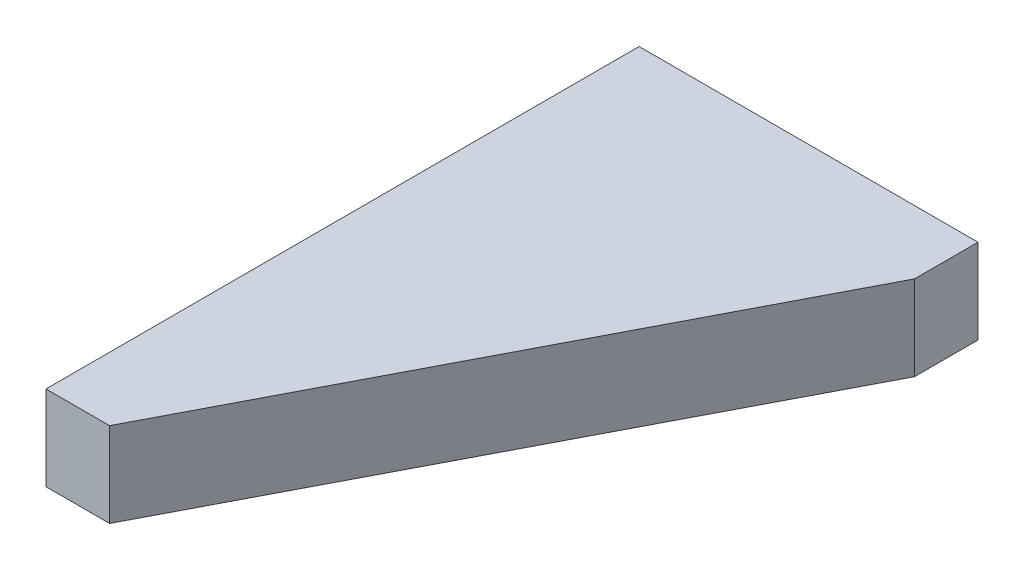
SolidWorks part; units mm, degrees
ref_plane "前视基准面" through (0, 0, 0) normal (0, 0, 1) x (1, 0, 0)
ref_plane "上视基准面" through (0, 0, 0) normal (0, 1, 0) x (1, 0, 0)
ref_plane "右视基准面" through (0, 0, 0) normal (1, 0, 0) x (0, 0, -1)
sketch "草图1" plane through (0, 0, 0) normal (0, 1, 0) x (1, 0, 0)
  line L1 (0, 0) -> (200, 0)
  line L2 (0, 0) -> (0, 140)
  line L3 (0, 140) -> (200, 140)
  line L4 (200, 0) -> (200, 140)
  dimension "D1" = 140
  dimension "D2" = 200
extrude "凸台-拉伸1" add sketch "草图1" along normal blind 20
sketch "草图3" plane through (0, 20, 0) normal (0, 1, 0) x (1, 0, 0)
  line L0 (0, 140) -> (80, 140)
  line L1 (200, 140) -> (0, 140) construction
  line L2 (80, 140) -> (80, 125)
  line L3 (80, 125) -> (15, 0)
  line L4 (0, 0) -> (200, 0) construction
  line L5 (15, 0) -> (0, 0)
  line L6 (0, 0) -> (0, 140)
  dimension "D1" = 15
  dimension "D2" = 15
  dimension "D3" = 80
extrude "切除-拉伸1" cut sketch "草图3" against normal through all flip side to cut
sketch "草图6" plane through (0, 0, 0) normal (-1, 0, 0) x (0, 0, 1)
  line L0 (-70, 0) -> (-70, 39.2152) construction
  line L1 (-140, 0) -> (0, 0) construction
  line L3 (0, 10) -> (-140, 10) construction
  line L4 (0, 20) -> (0, 0) construction
  line L5 (-140, 20) -> (-140, 0) construction
  point P0 (-120, 10)
  point P2 (-20, 10)
  dimension "D1" = 100
hole_wizard "M6 螺纹孔1" positions "草图6" profile "草图5" tap size "M6" standard "GB"
cosmetic thread "孔螺纹线1" parameters "D1"=12, "D2"=6
cosmetic thread "孔螺纹线2" parameters "D1"=12, "D2"=6
sketch "草图5" plane through (0, 10, -120) normal (0, 1, 0) x (0, 0, 1)
  line L0 (0, 0) -> (0, 16.5022)
  line L1 (0, 16.5022) -> (2.5, 15)
  line L2 (2.5, 15) -> (2.5, 0)
  line L5 (2.5, 0) -> (0, 0)
  line L10 (0, 16.5022) -> (-2.5, 15) construction
  line L11 (0, -6.35) -> (0, 107.95) construction
  dimension "螺纹孔钻头直径" = 5
  dimension "螺纹孔钻头深度" = 15
  dimension "导头角度" = 118
sketch "草图9" plane through (0, 0, -140) normal (0, 0, -1) x (-1, 0, 0)
  line L0 (-80, 10) -> (0, 10) construction
  line L1 (-80, 0) -> (-80, 20) construction
  line L2 (0, 20) -> (0, 0) construction
  line L4 (-40, 10) -> (-40, 33.5453) construction
  point P0 (-72.5, 10)
  point P2 (-7.5, 10)
  dimension "D1" = 65
hole_wizard "M6 螺纹孔2" positions "草图9" profile "草图8" tap size "M6" standard "GB"
sketch "草图8" plane through (72.5, 10, -140) normal (1, 0, 0) x (0, 1, 0)
  line L0 (0, 0) -> (0, 16.5022)
  line L1 (0, 16.5022) -> (2.5, 15)
  line L2 (2.5, 15) -> (2.5, 0)
  line L5 (2.5, 0) -> (0, 0)
  line L10 (0, 16.5022) -> (-2.5, 15) construction
  line L11 (0, -6.35) -> (0, 107.95) construction
  dimension "螺纹孔钻头直径" = 5
  dimension "螺纹孔钻头深度" = 15
  dimension "导头角度" = 118
cosmetic thread "孔螺纹线3" parameters "D1"=12, "D2"=6
cosmetic thread "孔螺纹线4" parameters "D1"=12, "D2"=6
